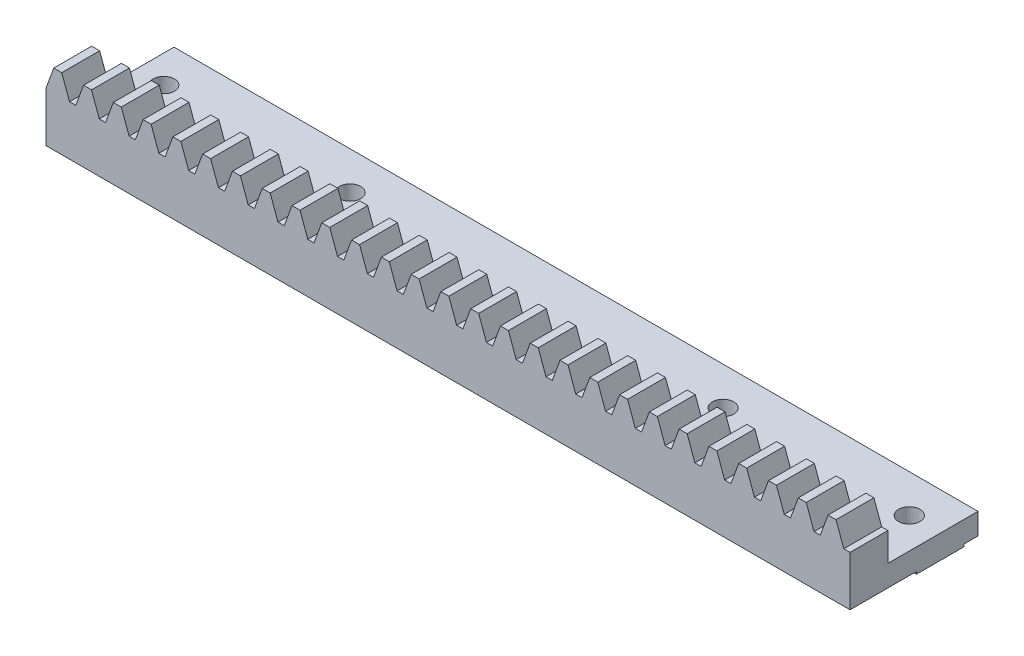
SolidWorks part; units mm, degrees
material "1.1193 (C45G)"
ref_plane "Front" through (0, 0, 0) normal (0, 0, 1) x (1, 0, 0)
ref_plane "Top" through (0, 0, 0) normal (0, 1, 0) x (1, 0, 0)
ref_plane "Right" through (0, 0, 0) normal (1, 0, 0) x (0, 0, -1)
sketch "Sketch1" plane through (0, 0, 0) normal (0, 0, 1) x (1, 0, 0)
  line L1 (0, 0) -> (169.646, 0)
  line L2 (0, 0) -> (0, -11)
  line L3 (0, -11) -> (169.646, -11)
  line L4 (169.646, 0) -> (169.646, -11)
  dimension "D1" = 11
  dimension "L" = 169.646
extrude "Extrude1" add sketch "Sketch1" along normal blind 27
sketch "Sketch2" plane through (0, 0, 27) normal (0, 0, 1) x (1, 0, 0)
  line L0 (0, 0) -> (1.6379, 4.5)
  line L1 (1.6379, 4.5) -> (3.3236, 4.5)
  line L2 (3.3236, 4.5) -> (4.9614, 0)
  line L3 (169.646, 0) -> (0, 0) construction
  line L4 (0, 0) -> (4.9614, 0)
  line L5 (0.9099, 2.5) -> (4.0515, 2.5) construction
  dimension "alpha2" = 70
  dimension "alpha" = 110
  dimension "ha" = 2
  dimension "hf" = 2.5
  dimension "S" = 3.1416
extrude "Extrude2" add sketch "Sketch2" against normal blind 8
pattern_linear "LPattern1" count 27 spacing 6.2832 along (1, 0, 0) of "Extrude2"
sketch "草图1" plane through (0, 0, 0) normal (0, 1, 0) x (1, 0, 0)
  line L0 (169.646, -27) -> (169.646, 0) construction
  line L1 (0, 0) -> (169.646, 0)
  line L2 (0, 0) -> (0, -19)
  line L3 (0, -19) -> (169.646, -19)
  line L4 (169.646, 0) -> (169.646, -19)
extrude "切除-拉伸1" cut sketch "草图1" against normal blind 6
sketch "草图2" plane through (0, -6, 0) normal (0, 1, 0) x (1, 0, 0)
  line L0 (0, 0) -> (0, -19) construction
  line L1 (10, -3) -> (41, -3)
  line L2 (10, -3) -> (10, -13)
  line L3 (10, -13) -> (41, -13)
  line L4 (41, -3) -> (41, -13)
  line L5 (169.646, 0) -> (0, 0) construction
  dimension "D1" = 10
  dimension "D2" = 3
  dimension "D3" = 31
  dimension "D4" = 10
extrude "凸台-拉伸1" [suppressed] add sketch "草图2" along normal blind 10.5
chamfer "倒角1" [suppressed] distance 10.5 distance2 10
fillet "圆角1" [suppressed] radius 1.5
pattern_linear "阵列(线性)1" [suppressed] count 2 spacing 118
sketch "草图3" plane through (0, -6, 0) normal (0, 1, 0) x (1, 0, 0)
  circle A0 centre (5.8571, -8) radius 2.25
  circle A1 centre (45.1429, -8) radius 2.25
  dimension "D1" = 4.5
  dimension "D3" = 4.5
extrude "切除-拉伸2" cut sketch "草图3" against normal blind 10.5
pattern_linear "阵列(线性)2" count 2 spacing 118 along (1, 0, 0) of "切除-拉伸2"
sketch "草图5" plane through (0, -11, 0) normal (0, -1, 0) x (1, 0, 0)
  line L0 (169.646, 27) -> (169.646, 0) construction
  line L1 (0, 27) -> (169.646, 27)
  line L2 (0, 27) -> (0, 13)
  line L3 (0, 13) -> (169.646, 13)
  line L4 (169.646, 27) -> (169.646, 13)
  line L5 (0, 27) -> (0, 0) construction
  line L6 (169.646, 0) -> (0, 0)
  line L7 (169.646, 0) -> (169.646, 3)
  line L8 (169.646, 3) -> (0, 3)
  line L9 (0, 0) -> (0, 3)
  circle A0 centre (5.8571, 8) radius 2.25 construction
  dimension "D2" = 5
  dimension "D1" = 5
extrude "切除-拉伸3" cut sketch "草图5" against normal blind 0.5
